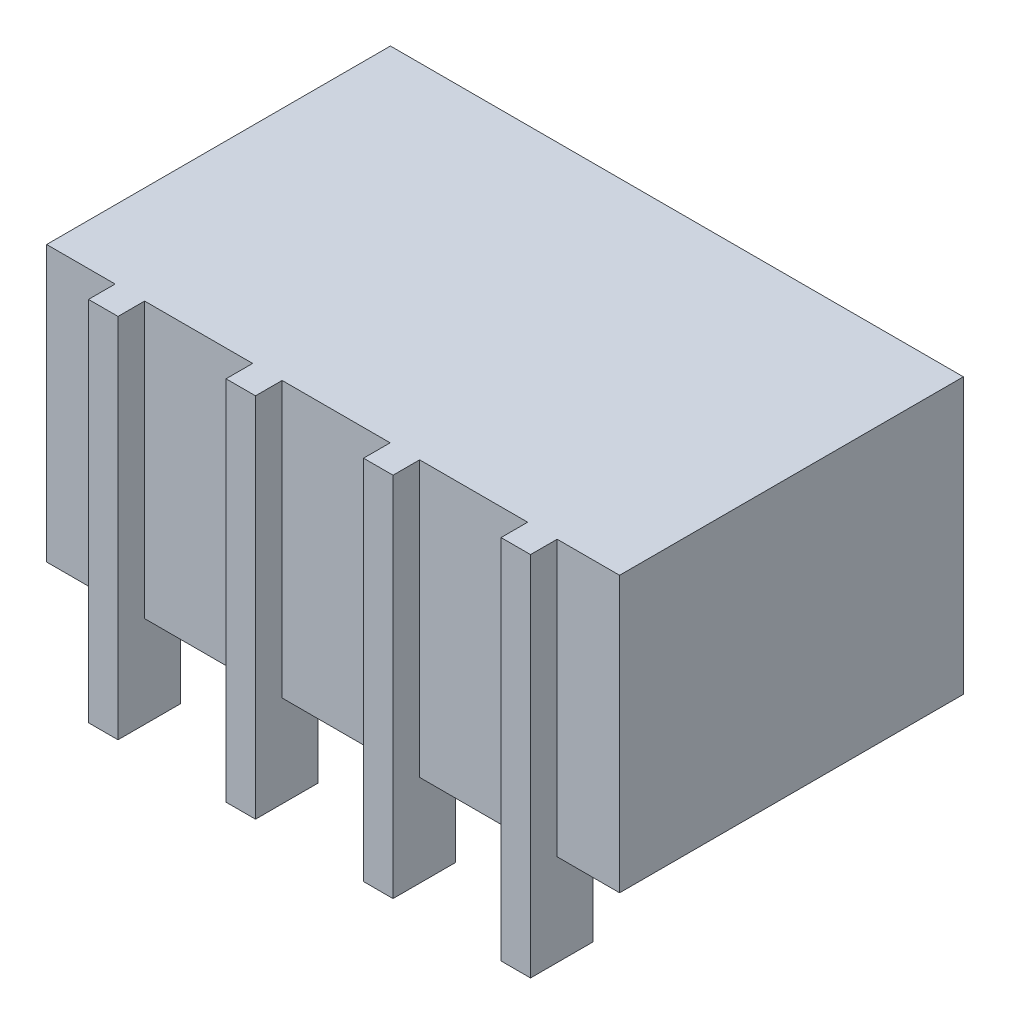
SolidWorks part; units mm, degrees
ref_plane "前视基准面" through (0, 0, 0) normal (0, 0, 1) x (1, 0, 0)
ref_plane "上视基准面" through (0, 0, 0) normal (0, 1, 0) x (1, 0, 0)
ref_plane "右视基准面" through (0, 0, 0) normal (1, 0, 0) x (0, 0, -1)
sketch "草图1" plane through (0, 0, 0) normal (0, 0, 1) x (1, 0, 0)
  line L1 (11.283, -1.3864) -> (-1.217, -1.3864)
  line L2 (11.283, -1.3864) -> (11.283, 4.6136)
  line L3 (11.283, 4.6136) -> (-1.217, 4.6136)
  line L4 (-1.217, -1.3864) -> (-1.217, 4.6136)
  dimension "D1" = 12.5
  dimension "D2" = 6
extrude "拉伸1" add sketch "草图1" along normal blind 7.5
sketch "草图2" plane through (0, 0, 0) normal (0, 0, -1) x (-1, 0, 0)
  line L1 (-10.7762, -0.509) -> (0.5667, -0.509)
  line L2 (-10.7762, -0.509) -> (-10.7762, 3.9681)
  line L3 (-10.7762, 3.9681) -> (0.5667, 3.9681)
  line L4 (0.5667, -0.509) -> (0.5667, 3.9681)
  circle A0 centre (-7.9863, 2.1919) radius 0.4804
  circle A1 centre (-6.3347, 2.1919) radius 0.5172
  circle A2 centre (-4.2993, 2.1919) radius 0.5827
  circle A3 centre (-2.2306, 2.1919) radius 0.5005
extrude "切除-拉伸1" cut sketch "草图2" against normal blind 5
sketch "草图3" plane through (0, 4.6136, 4.8864) normal (0, -1, 0) x (1, 0, 0)
  line L0 (6.9207, 1.8301) -> (6.2773, 1.8301)
  line L1 (9.9207, 1.8301) -> (9.2773, 1.8301)
  line L2 (9.9207, 1.8301) -> (9.9207, 3.1942)
  line L3 (9.9207, 3.1942) -> (9.2773, 3.1942)
  line L4 (9.2773, 1.8301) -> (9.2773, 3.1942)
  line L5 (6.9207, 1.8301) -> (6.9207, 3.1942)
  line L6 (6.9207, 3.1942) -> (6.2773, 3.1942)
  line L7 (6.2773, 1.8301) -> (6.2773, 3.1942)
  line L8 (3.9207, 1.8301) -> (3.2773, 1.8301)
  line L9 (3.9207, 1.8301) -> (3.9207, 3.1942)
  line L10 (3.9207, 3.1942) -> (3.2773, 3.1942)
  line L11 (3.2773, 1.8301) -> (3.2773, 3.1942)
  line L12 (0.9207, 1.8301) -> (0.2773, 1.8301)
  line L13 (0.9207, 1.8301) -> (0.9207, 3.1942)
  line L14 (0.9207, 3.1942) -> (0.2773, 3.1942)
  line L15 (0.2773, 1.8301) -> (0.2773, 3.1942)
extrude "拉伸2" add sketch "草图3" along normal blind 8
